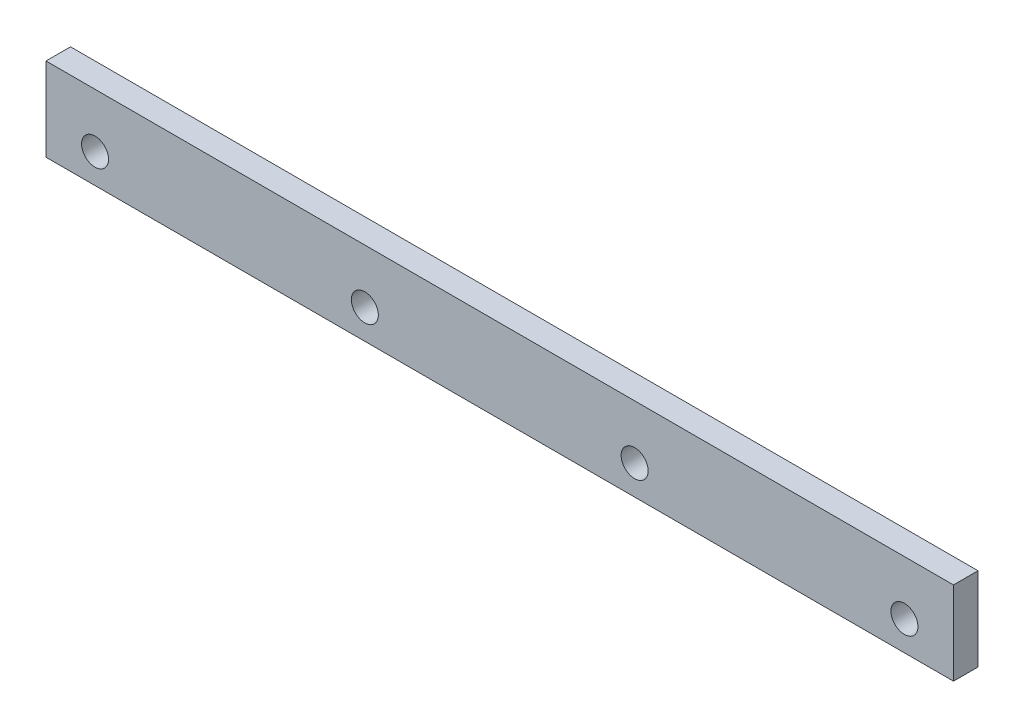
SolidWorks part; units mm, degrees
ref_plane "前视基准面" through (0, 0, 0) normal (0, 0, 1) x (1, 0, 0)
ref_plane "上视基准面" through (0, 0, 0) normal (0, 1, 0) x (1, 0, 0)
ref_plane "右视基准面" through (0, 0, 0) normal (1, 0, 0) x (0, 0, -1)
other "Configuration Table"
sketch "草图1" plane through (0, 0, 0) normal (0, 0, 1) x (1, 0, 0)
  line L0 (165, -5) -> (55, -5) construction
  line L1 (-185, -17) -> (185, -17)
  line L2 (-185, -17) -> (-185, 17)
  line L3 (-185, 17) -> (185, 17)
  line L4 (185, -17) -> (185, 17)
  line L5 (0, 17) -> (0, -17) construction
  line L6 (-185, 0) -> (185, 0) construction
  circle A0 centre (165, -5) radius 5.5
  circle A1 centre (55, -5) radius 5.5
  circle A2 centre (-55, -5) radius 5.5
  circle A3 centre (-165, -5) radius 5.5
  point P0 (0, 0)
  dimension "D3" = 11
  dimension "D1" = 370
  dimension "D2" = 34
  dimension "D4" = 12
  dimension "D5" = 20
  dimension "D7" = 110
  dimension "D6" = 4
extrude "凸台-拉伸1" add sketch "草图1" along normal blind 10
